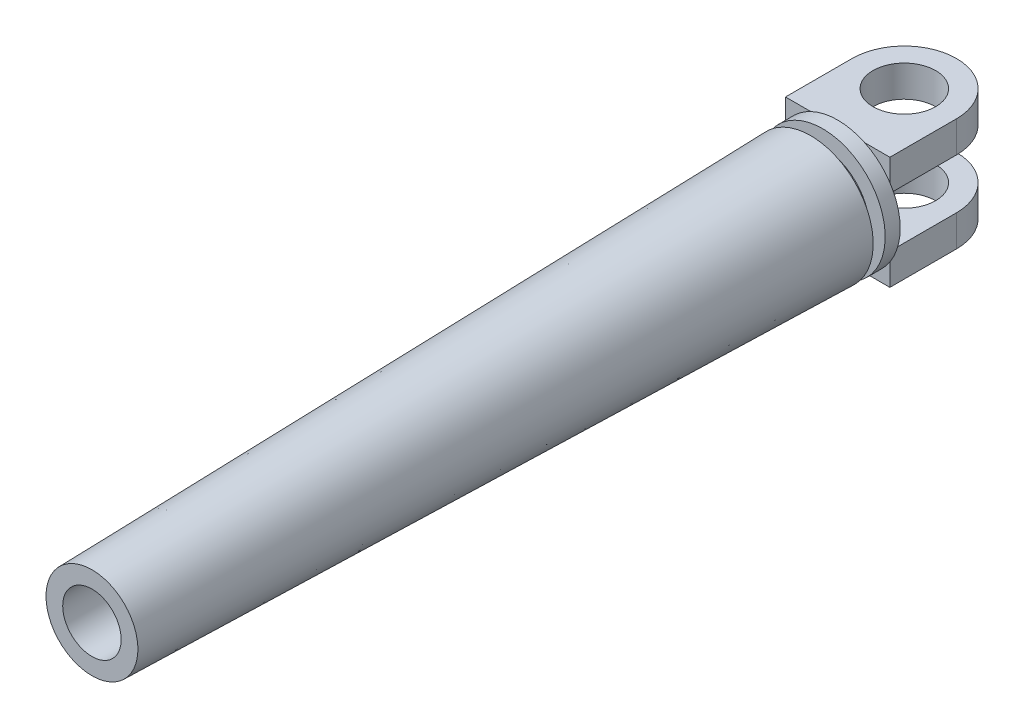
SolidWorks part; units mm, degrees
ref_plane "Front Plane" through (0, 0, 0) normal (0, 0, 1) x (1, 0, 0)
ref_plane "Top Plane" through (0, 0, 0) normal (0, 1, 0) x (1, 0, 0)
ref_plane "Right Plane" through (0, 0, 0) normal (1, 0, 0) x (0, 0, -1)
other "Configuration Table"
sketch "Sketch2" plane through (0, 0, 0) normal (0, 1, 0) x (1, 0, 0)
  line L0 (0, 0) -> (0, -31.9129) construction
  line L1 (25, 0) -> (25, -31.9129)
  line L2 (-25, 0) -> (-25, -31.9129)
  line L3 (-25, -31.9129) -> (25, -31.9129)
  circle A0 centre (0, 0) radius 15
  arc A1 (25, 0) -> (-25, 0) centre (0, 0) ccw
  point P3 (0, -15.9565)
  dimension "D1" = 30
  dimension "D2" = 25
extrude "Boss-Extrude1" add sketch "Sketch2" along normal blind 15
ref_plane "Plane1" through (0, -12, 0) normal (0, -1, 0) x (-1, 0, 0)
sketch "Sketch3" plane through (0, 0, 31.9129) normal (0, 0, 1) x (1, 0, 0)
  line L0 (0, 15) -> (0, -12) construction
  line L1 (-25, 15) -> (25, 15) construction
  line L2 (-27.5, -12) -> (27.5, -12) construction
sketch "Sketch4" plane through (0, -12, 0) normal (0, -1, 0) x (-1, 0, 0)
  line L0 (0, -31.9129) -> (29.9332, -31.9129)
  line L1 (25, -31.9129) -> (-25, -31.9129) construction
  line L2 (29.9332, -31.9129) -> (29.9332, -39.0865)
  line L3 (29.9332, -39.0865) -> (22.3827, -39.0865)
  line L4 (22.3827, -39.0865) -> (22.3827, -44.8425)
  line L5 (22.3827, -44.8425) -> (29.9332, -44.8425)
  line L6 (29.9332, -44.8425) -> (22, -389.0865)
  line L7 (0, -31.9129) -> (0, -39.0865)
  line L8 (0, -39.0865) -> (14, -39.0865)
  line L9 (14, -39.0865) -> (14, -389.0865)
  line L10 (14, -389.0865) -> (22, -389.0865)
  dimension "D1" = 350
  dimension "D2" = 14
  dimension "D3" = 8
revolve "Revolve1" add sketch "Sketch4" angle 360 about L7
mirror "Mirror5" about plane through (0, -12, 0) normal (0, -1, 0) of "Boss-Extrude1"
